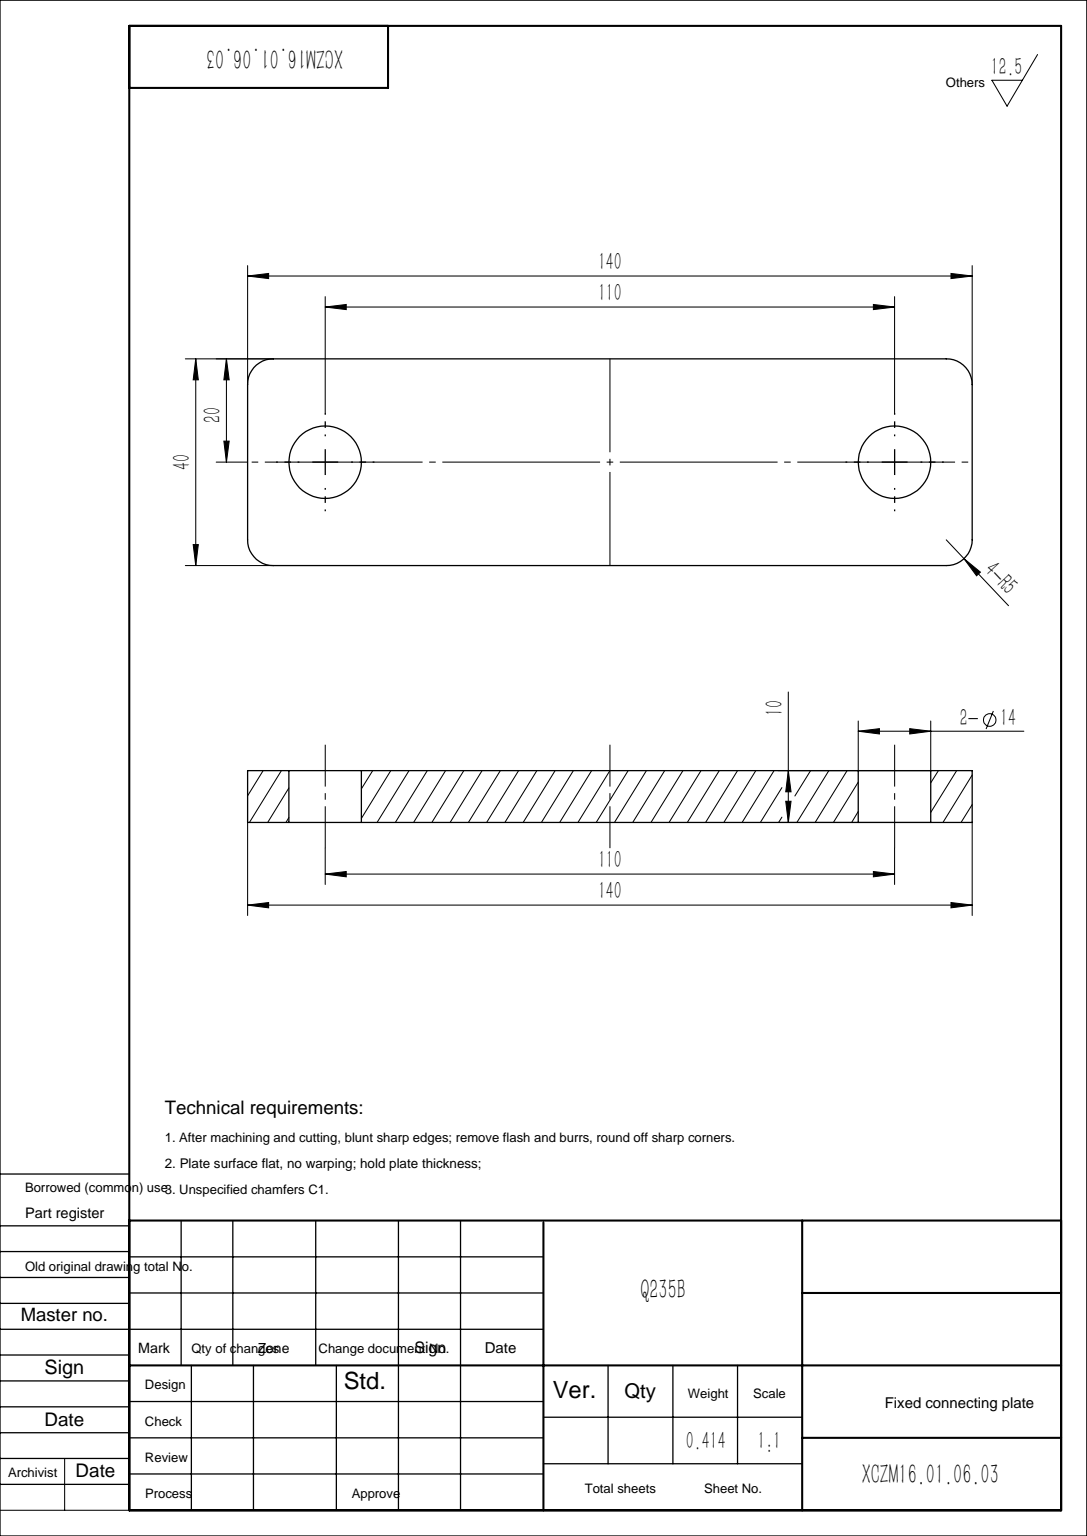
SolidWorks part; units mm, degrees
material "Q235B"
ref_plane "Front Plane" through (0, 0, 0) normal (0, 0, 1) x (1, 0, 0)
ref_plane "Top Plane" through (0, 0, 0) normal (0, 1, 0) x (1, 0, 0)
ref_plane "Right Plane" through (0, 0, 0) normal (1, 0, 0) x (0, 0, -1)
sketch "Sketch2" plane through (0, 0, 0) normal (0, 1, 0) x (1, 0, 0)
  line L0 (0, 20) -> (0, -20) construction
  line L1 (65, -20) -> (-65, -20)
  line L2 (70, -15) -> (70, 15)
  line L3 (65, 20) -> (-65, 20)
  line L4 (-70, -15) -> (-70, 15)
  line L5 (70, -20) -> (-70, 20) construction
  line L6 (70, 20) -> (-70, -20) construction
  arc A0 (-65, -20) -> (-70, -15) centre (-65, -15) cw
  arc A1 (70, 15) -> (65, 20) centre (65, 15) ccw
  arc A2 (65, -20) -> (70, -15) centre (65, -15) ccw
  arc A3 (-65, 20) -> (-70, 15) centre (-65, 15) ccw
  circle A4 centre (-55, 0) radius 7
  circle A5 centre (55, 0) radius 7
  point P0 (0, 0)
  dimension "D3" = 5
  dimension "D4" = 14
  dimension "D5" = 110
  dimension "D1" = 40
  dimension "D2" = 140
extrude "Boss-Extrude1" add sketch "Sketch2" along normal blind 10
